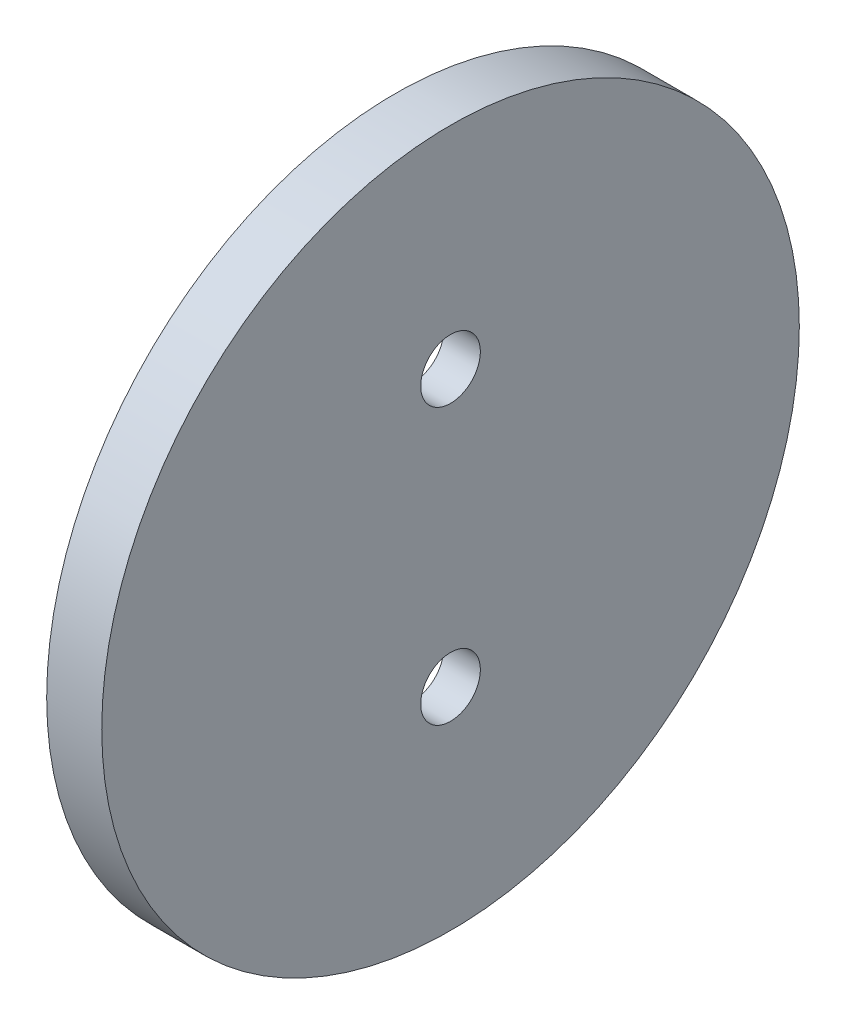
from build123d import *

# Parameters (mm, degrees)
SKETCH2_R          = 3.25
CUT_EXTRUDE1_DEPTH = 55.074023338


with BuildPart() as part:
    # Sketch1 → Revolve1 (revolve)
    with BuildSketch(Plane.XY, mode=Mode.PRIVATE) as revolve1_sk:
        Polygon((0, 0), (0, 38), (-6, 38), (-6, 33), (-4, 33), (-4, 0), align=None)
    revolve(revolve1_sk.sketch.rotate(Axis((0, 0, 0), (-1, 0, 0)), 90), axis=Axis((0, 0, 0), (-1, 0, 0)))

    # Sketch2 → Cut-Extrude1 (cut, through all)
    with BuildSketch(Plane(origin=(0, 0, 0), x_dir=(0, 0, -1), z_dir=(1, 0, 0))):
        with Locations((0, 15)):
            Circle(SKETCH2_R)
        with Locations((0, -15)):
            Circle(SKETCH2_R)
    extrude(amount=-CUT_EXTRUDE1_DEPTH, mode=Mode.SUBTRACT)


solid = part.part
